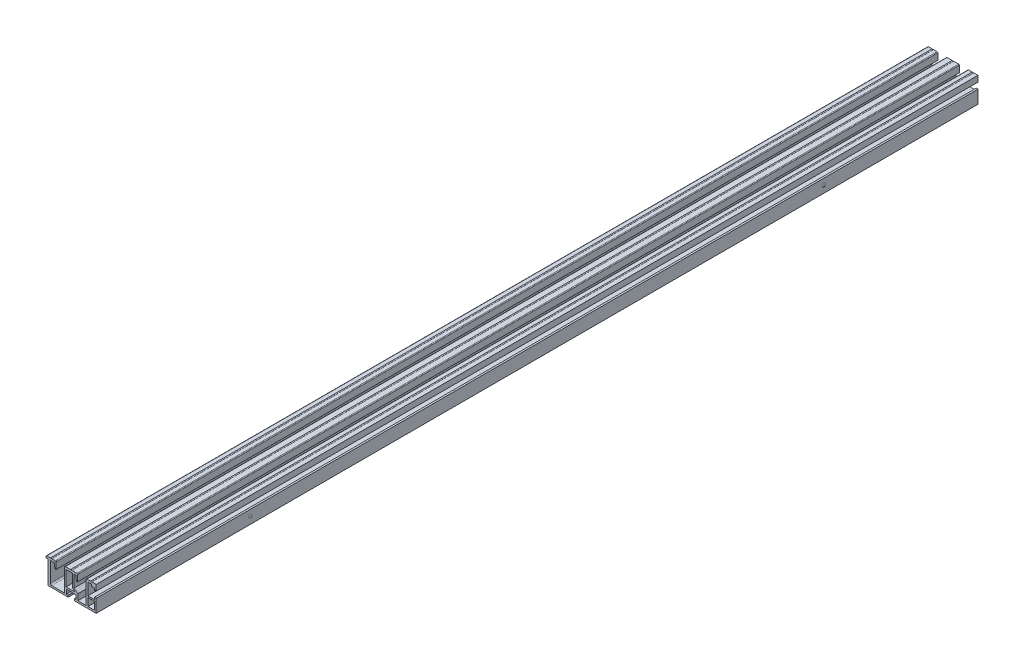
from build123d import *

# Parameters (mm, degrees)
SKETCH_1_W               = 9
SKETCH_1_H               = 11
EXTRUDE_1_DEPTH          = 615
CUT_EXTRUDE_1_DEPTH      = 620.823563605
CUT_EXTRUDE_1_DEPTH_BACK = 620.823563605
SKETCH_3_R               = 2.5
CUT_EXTRUDE_2_DEPTH      = 0.1


with BuildPart() as part:
    # 草图1 → 凸台-拉伸1 (new, symmetric)
    with BuildSketch(Plane.XY):
        with BuildLine():
            Line((-28.5, 32), (-27.5, 25))
            Line((-27.5, 25), (-26, 25))
            Line((-26, 25), (-26, 34))
            ThreePointArc((-26, 34), (-26.292893219, 34.707106781), (-27, 35))
            Line((-27, 35), (-34.1, 35))
            ThreePointArc((-34.1, 35), (-35, 34.7), (-35.9, 35))
            Line((-35.9, 35), (-43, 35))
            ThreePointArc((-43, 35), (-43.707106781, 34.707106781), (-44, 34))
            Line((-44, 34), (-44, 2.5))
            Line((-44, 2.5), (-62, 2.5))
            ThreePointArc((-62, 2.5), (-63.414213562, 3.085786438), (-64, 4.5))
            Line((-64, 4.5), (-64, 31))
            ThreePointArc((-64, 31), (-63.707106781, 31.707106781), (-63, 32))
            Line((-63, 32), (-58.5, 32))
            Line((-58.5, 32), (-57.5, 25))
            Line((-57.5, 25), (-56, 25))
            Line((-56, 25), (-56, 34))
            ThreePointArc((-56, 34), (-56.292893219, 34.707106781), (-57, 35))
            Line((-57, 35), (-62.1, 35))
            ThreePointArc((-62.1, 35), (-63, 34.7), (-63.9, 35))
            Line((-63.9, 35), (-69, 35))
            ThreePointArc((-69, 35), (-69.707106781, 34.707106781), (-70, 34))
            Line((-70, 34), (-70, 32))
            Line((-70, 32), (-68, 32))
            ThreePointArc((-68, 32), (-67.292893219, 31.707106781), (-67, 31))
            Line((-67, 31), (-67, 0))
            Line((-67, 0), (-39, 0))
            Line((-39, 0), (-39, 2.5))
            Line((-39, 2.5), (-41.5, 2.5))
            Line((-41.5, 2.5), (-41.5, 8.5))
            Line((-41.5, 8.5), (-28.006, 8.5))
            Line((-28.006, 8.5), (-28.006, 2.5))
            Line((-28.006, 2.5), (-30.5, 2.5))
            Line((-30.5, 2.5), (-30.5, 0))
            Line((-30.5, 0), (0, 0))
            Line((0, 0), (0, 18.25))
            Line((0, 18.25), (-2.5, 18.25))
            Line((-2.5, 18.25), (-2.5, 15.5))
            Line((-2.5, 15.5), (-11.5, 15.5))
            Line((-11.5, 15.5), (-11.5, 31))
            ThreePointArc((-11.5, 31), (-11.207106781, 31.707106781), (-10.5, 32))
            Line((-10.5, 32), (-6.5, 32))
            Line((-6.5, 32), (-6.5, 29.5))
            Line((-6.5, 29.5), (-2.5, 29.5))
            Line((-2.5, 29.5), (-2.5, 26.75))
            Line((-2.5, 26.75), (0, 26.75))
            Line((0, 26.75), (0, 35))
            Line((0, 35), (-6.1, 35))
            ThreePointArc((-6.1, 35), (-7, 34.7), (-7.9, 35))
            Line((-7.9, 35), (-13, 35))
            ThreePointArc((-13, 35), (-13.707106781, 34.707106781), (-14, 34))
            Line((-14, 34), (-14, 2.5))
            Line((-14, 2.5), (-25.5, 2.5))
            Line((-25.5, 2.5), (-25.5, 11))
            Line((-25.5, 11), (-31, 15))
            Line((-31, 15), (-31, 32))
            Line((-31, 32), (-28.5, 32))
        make_face()
        with Locations((-7, 8)):
            Rectangle(SKETCH_1_W, SKETCH_1_H, mode=Mode.SUBTRACT)
        with BuildLine():
            Line((-42, 11), (-42, 32))
            Line((-42, 32), (-33, 32))
            Line((-33, 32), (-33, 13.981550817))
            Line((-33, 13.981550817), (-30.143873685, 11.904368042))
            ThreePointArc((-30.143873685, 11.904368042), (-29.962468198, 11.345377914), (-30.437959534, 11))
            Line((-30.437959534, 11), (-42, 11))
        make_face(mode=Mode.SUBTRACT)
    extrude(amount=EXTRUDE_1_DEPTH, both=True)

    # 草图2 → 切除-拉伸1 (cut, two sides: drawn at the far end of the back side and taken through both)
    with BuildSketch(Plane(origin=(0, 2.5, 0), x_dir=(1, 0, 0), z_dir=(0, 1, 0)).offset(-CUT_EXTRUDE_1_DEPTH_BACK)):
        with BuildLine():
            Line((-15.5, -230.5), (-15.5, -189.5))
            ThreePointArc((-15.5, -189.5), (-20, -185), (-24.5, -189.5))
            Line((-24.5, -189.5), (-24.5, -230.5))
            ThreePointArc((-24.5, -230.5), (-20, -235), (-15.5, -230.5))
        make_face()
        with BuildLine():
            Line((-45.5, 95.5), (-45.5, 54.5))
            ThreePointArc((-45.5, 54.5), (-50, 50), (-54.5, 54.5))
            Line((-54.5, 54.5), (-54.5, 95.5))
            ThreePointArc((-54.5, 95.5), (-50, 100), (-45.5, 95.5))
        make_face()
        with BuildLine():
            Line((-45.5, -95.5), (-45.5, -54.5))
            ThreePointArc((-45.5, -54.5), (-50, -50), (-54.5, -54.5))
            Line((-54.5, -54.5), (-54.5, -95.5))
            ThreePointArc((-54.5, -95.5), (-50, -100), (-45.5, -95.5))
        make_face()
        with BuildLine():
            Line((-15.5, 230.5), (-15.5, 189.5))
            ThreePointArc((-15.5, 189.5), (-20, 185), (-24.5, 189.5))
            Line((-24.5, 189.5), (-24.5, 230.5))
            ThreePointArc((-24.5, 230.5), (-20, 235), (-15.5, 230.5))
        make_face()
    extrude(amount=CUT_EXTRUDE_1_DEPTH + CUT_EXTRUDE_1_DEPTH_BACK, mode=Mode.SUBTRACT)

    # 草图3 → 切除-拉伸2 (cut)
    with BuildSketch(Plane(origin=(0, 0, 0), x_dir=(0, 0, -1), z_dir=(1, 0, 0))):
        with Locations((-400, 10)):
            Circle(SKETCH_3_R)
        with Locations(Location((400, 10, 0), (0, 0, 180))):
            Circle(SKETCH_3_R)
    extrude(amount=-CUT_EXTRUDE_2_DEPTH, mode=Mode.SUBTRACT)


solid = part.part
